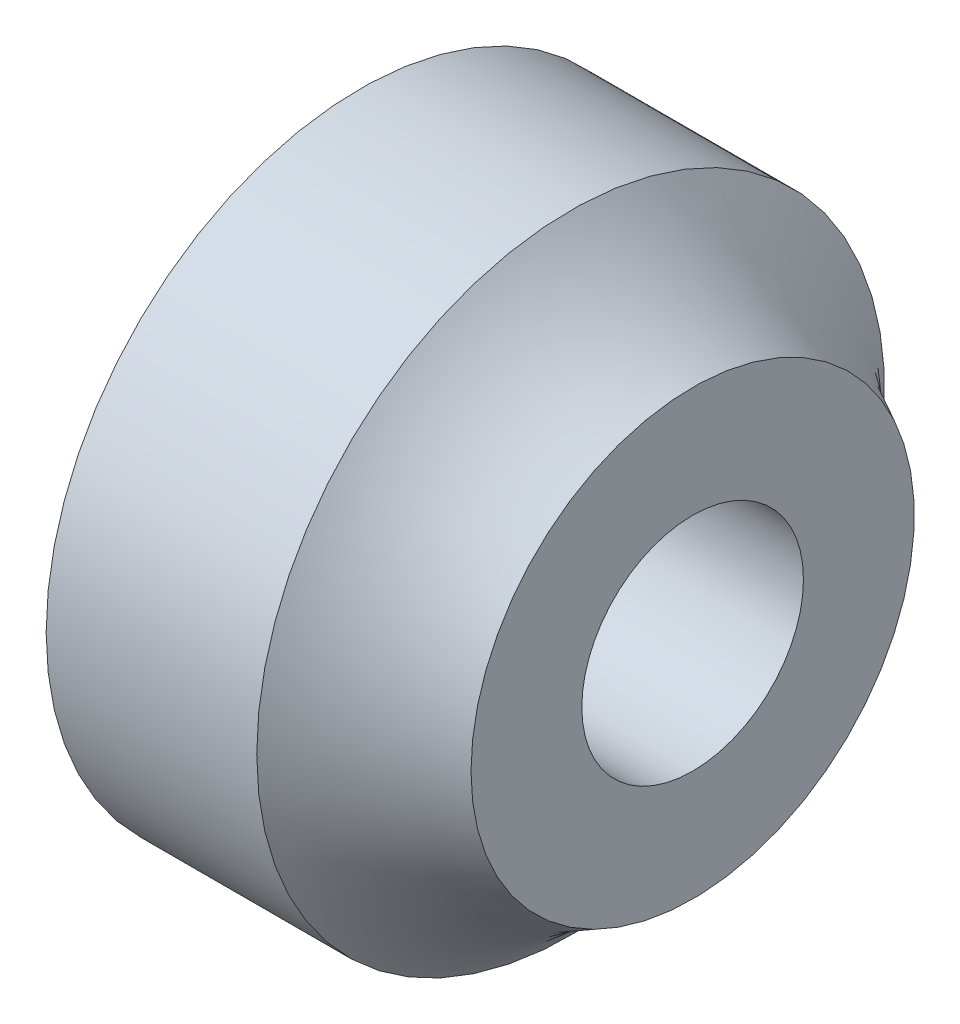
from build123d import *

# Parameters (mm, degrees)
CUT_EXTRUDE1_DEPTH      = 31.033314835
CUT_EXTRUDE1_DEPTH_BACK = 31.033314835
SKETCH2_R               = 6


with BuildPart() as part:
    # Sketch1 → Revolve1 (revolve)
    with BuildSketch(Plane.XY, mode=Mode.PRIVATE) as revolve1_sk:
        with BuildLine():
            Line((0, 0), (0, 17))
            Line((0, 17), (11.4, 17))
            ThreePointArc((11.4, 17), (14.400024627, 14.104032508), (18, 12))
            Line((18, 12), (18, 0))
            Line((18, 0), (0, 0))
        make_face()
    revolve(revolve1_sk.sketch.rotate(Axis((0, 0, 0), (1, 0, 0)), 90), axis=Axis((0, 0, 0), (1, 0, 0)))

    # Sketch2 → Cut-Extrude1 (cut, two sides: drawn at the far end of the back side and taken through both)
    with BuildSketch(Plane(origin=(18, 0, 0), x_dir=(0, 0, -1), z_dir=(1, 0, 0)).offset(-CUT_EXTRUDE1_DEPTH_BACK)):
        Circle(SKETCH2_R)
    extrude(amount=CUT_EXTRUDE1_DEPTH + CUT_EXTRUDE1_DEPTH_BACK, mode=Mode.SUBTRACT)


solid = part.part
